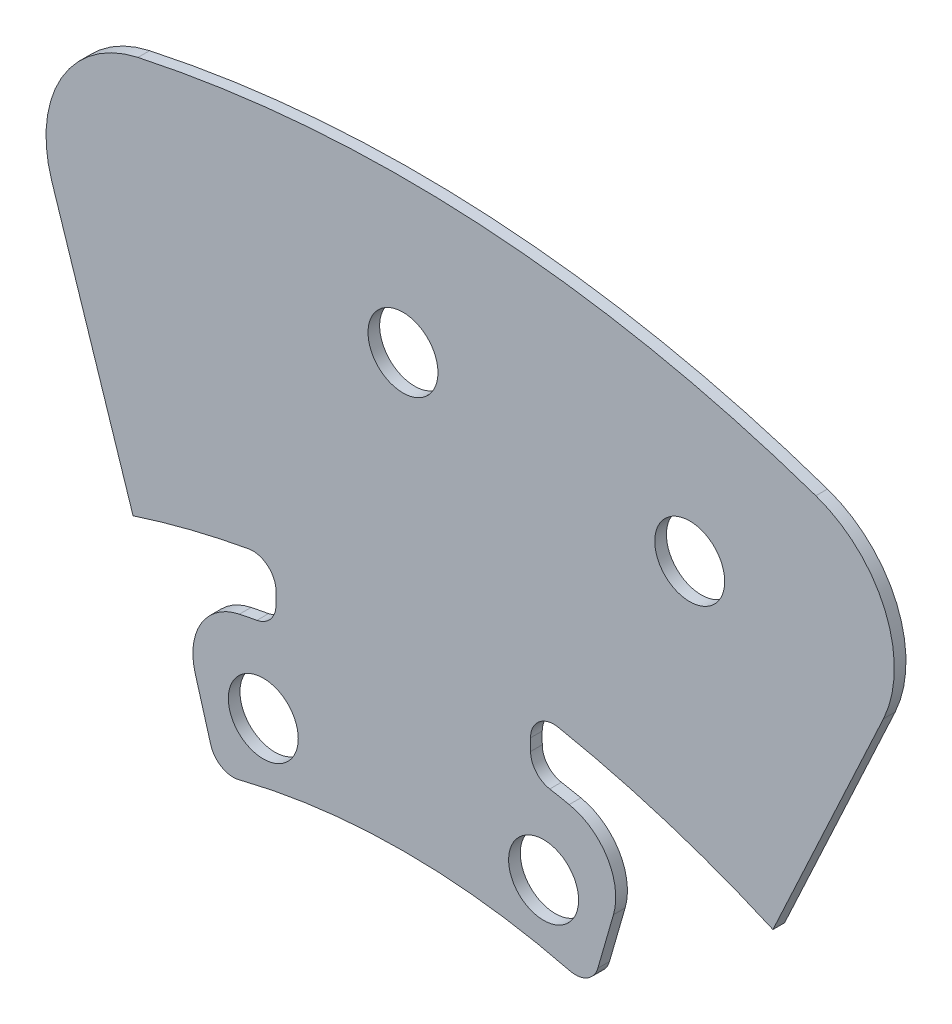
SolidWorks part; units mm, degrees
ref_plane "Front Plane" through (0, 0, 0) normal (0, 0, 1) x (1, 0, 0)
ref_plane "Top Plane" through (0, 0, 0) normal (0, 1, 0) x (1, 0, 0)
ref_plane "Right Plane" through (0, 0, 0) normal (1, 0, 0) x (0, 0, -1)
other "Configuration Table"
sketch "Sketch1" plane through (0, 0, 0) normal (0, 0, 1) x (1, 0, 0)
  line L0 (-23.148, -8.7302) -> (-30.1228, 12.6492)
  line L1 (-16.4845, -22.4079) -> (-17.8243, -17.7563)
  line L2 (16.7111, -22.4079) -> (18.051, -17.7563)
  line L3 (-10.8867, -8.1986) -> (-10.8867, -9.2151)
  line L4 (31.7286, -12.0209) -> (41.2083, 8.3718)
  line L5 (10.9419, -8.1726) -> (10.9443, -9.1891)
  arc A0 (35.4082, 22.0381) -> (-22.7312, 25.5245) centre (0.1133, -80.0318) ccw
  arc A1 (-13.2428, -6.2306) -> (-23.148, -8.7302) centre (0.1133, -80.0318) ccw
  arc A2 (-22.7312, 25.5245) -> (-30.1228, 12.6492) centre (-20.616, 15.7508) ccw
  arc A3 (18.051, -17.7563) -> (14.2565, -11.4755) centre (13.2463, -16.3723) ccw
  arc A4 (-14.0299, -11.4755) -> (-17.8243, -17.7563) centre (-13.0197, -16.3723) ccw
  circle A5 centre (12.0605, -18.175) radius 3
  circle A6 centre (-11.9814, -18.2037) radius 3
  arc A7 (14.3001, -23.7936) -> (-14.0734, -23.7936) centre (0.1133, -80.0318) ccw
  arc A8 (-16.4845, -22.4079) -> (-14.0734, -23.7936) centre (-14.5626, -21.8543) ccw
  arc A9 (14.3001, -23.7936) -> (16.7111, -22.4079) centre (14.7893, -21.8543) ccw
  arc A10 (10.9443, -9.1891) -> (12.5879, -11.1523) centre (12.9443, -9.1843) ccw
  arc A11 (13.2934, -6.199) -> (10.9419, -8.1726) centre (12.9419, -8.1678) ccw
  arc A12 (-10.8867, -8.1986) -> (-13.2428, -6.2306) centre (-12.8867, -8.1986) ccw
  arc A13 (-12.5256, -11.1823) -> (-14.0299, -11.4755) centre (0.1133, -80.0318) ccw
  arc A14 (-12.5256, -11.1823) -> (-10.8867, -9.2151) centre (-12.8867, -9.2151) ccw
  circle A15 centre (0, 14.9681) radius 3
  arc A16 (31.7286, -12.0209) -> (13.2934, -6.199) centre (-3.6729, -92.0208) ccw
  arc A17 (14.2565, -11.4755) -> (12.5879, -11.1523) centre (0.1133, -80.0318) ccw
  circle A18 centre (24.5917, 11.7604) radius 3
  arc A19 (41.2083, 8.3718) -> (35.4082, 22.0381) centre (32.1402, 12.5872) ccw
extrude "Boss-Extrude2" add sketch "Sketch1" along normal blind 1 contours L5 A10 A17 A3 L2 A9 A7 A8 L1 A4 A13 A14 L3 A12 A1 L0 A2 A0 A19 L4 A16 A11
